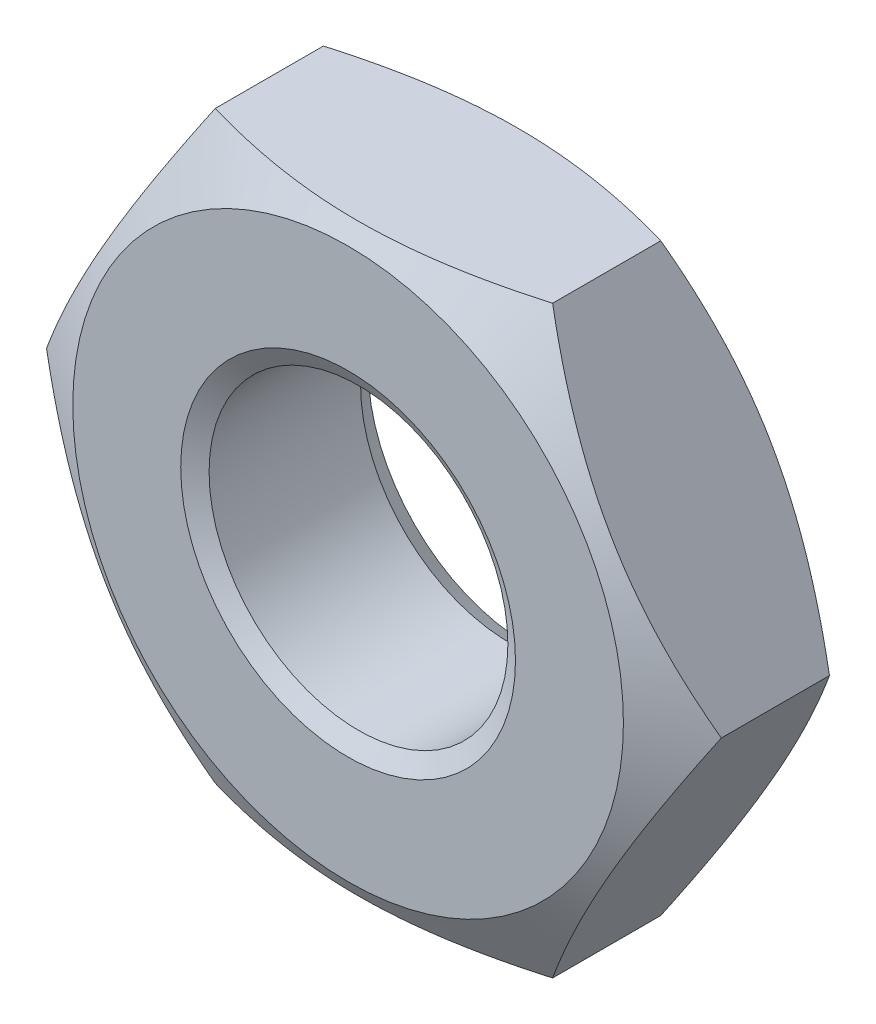
SolidWorks part; units mm, degrees
ref_plane "Front" through (0, 0, 0) normal (0, 0, 1) x (1, 0, 0)
ref_plane "Top" through (0, 0, 0) normal (0, 1, 0) x (1, 0, 0)
ref_plane "Right" through (0, 0, 0) normal (1, 0, 0) x (0, 0, -1)
sketch "Sketch1" plane through (0, 0, 0) normal (0, 0, 1) x (1, 0, 0)
  line L1 (3.7528, -6.5) -> (7.5056, 0)
  line L2 (7.5056, 0) -> (3.7528, 6.5)
  line L3 (3.7528, 6.5) -> (-3.7528, 6.5)
  line L4 (-3.7528, 6.5) -> (-7.5056, 0)
  line L5 (-7.5056, 0) -> (-3.7528, -6.5)
  line L6 (-3.7528, -6.5) -> (3.7528, -6.5)
  circle A0 centre (0, 0) radius 6.5 construction
  circle A1 centre (0, 0) radius 3.3235
  dimension "D" = 6.647
  dimension "s" = 13
extrude "BaseNut" add sketch "Sketch1" against normal blind 4
cosmetic thread "ThreadCosmetic1" parameters "D"=8
sketch "Sketch2" plane through (0, 0, 0) normal (0, 1, 0) x (1, 0, 0)
  line L0 (-7.5056, 4) -> (-6.125, 4)
  line L2 (-6.125, 4) -> (-7.5056, 3.2029)
  line L3 (-7.5056, 3.2029) -> (-7.5056, 4)
  line L4 (0, 3.3759) -> (0, -9.8171) construction
  line L6 (-9.7712, 2) -> (9.8853, 2) construction
  line L7 (-7.5056, 0.7971) -> (-7.5056, 0)
  line L8 (-6.125, 0) -> (-7.5056, 0.7971)
  line L9 (-7.5056, 0) -> (-6.125, 0)
  dimension "D1" = 30
  dimension "dw" = 12.25
  dimension "D2" = 2
revolve "Double-Chamfer" cut sketch "Sketch2" angle 360 about L4
chamfer "EndChamfer" distance 0.4 angle 30 2 edges at (3.3235, 0, -4) (3.3235, 0, 0)
sketch "Sketch3" plane through (0, 0, 0) normal (0, 1, 0) x (1, 0, 0)
  line L0 (0, 6.7075) -> (0, -2.1252) construction
  line L1 (2.647, 3.9383) -> (3.3235, 3.9383)
  line L2 (3.3235, 3.9383) -> (3.9094, 3.6)
  line L3 (3.9094, 3.6) -> (3.3235, 3.2618)
  line L4 (3.3235, 3.2618) -> (2.647, 3.2618)
  line L5 (2.647, 3.2618) -> (2.647, 3.9383)
  line L6 (3.3235, 3.6) -> (-3.3235, 3.6) construction
  dimension "D1" = 0.6765
  dimension "D2" = 6.647
revolve "Cut-Revolve10" [suppressed] cut sketch "Sketch3" angle 360 about L0
pattern_linear "LPattern10" [suppressed] count 4 spacing 0.8118 along (0, 0, 1)
equation "\"dw@Sketch2\" = \"s@Sketch1\"-0.75"
equation "\"D2@Sketch2\" = \"m@BaseNut\" / 2"
equation "\"D1@EndChamfer\" = \"m@BaseNut\" / 10"
equation "\"D2@Sketch3\" = \"D@Sketch1\""
equation "\"D1@Sketch3\" = (  \"D@ThreadCosmetic1\" - \"D@Sketch1\" )  / 2"
equation "\"D3@LPattern10\" = \"D1@Sketch3\" * 1.2"
equation "\"D1@LPattern10\" = (  \"m@BaseNut\" - \"D1@EndChamfer\" )  / \"D3@LPattern10\" "
